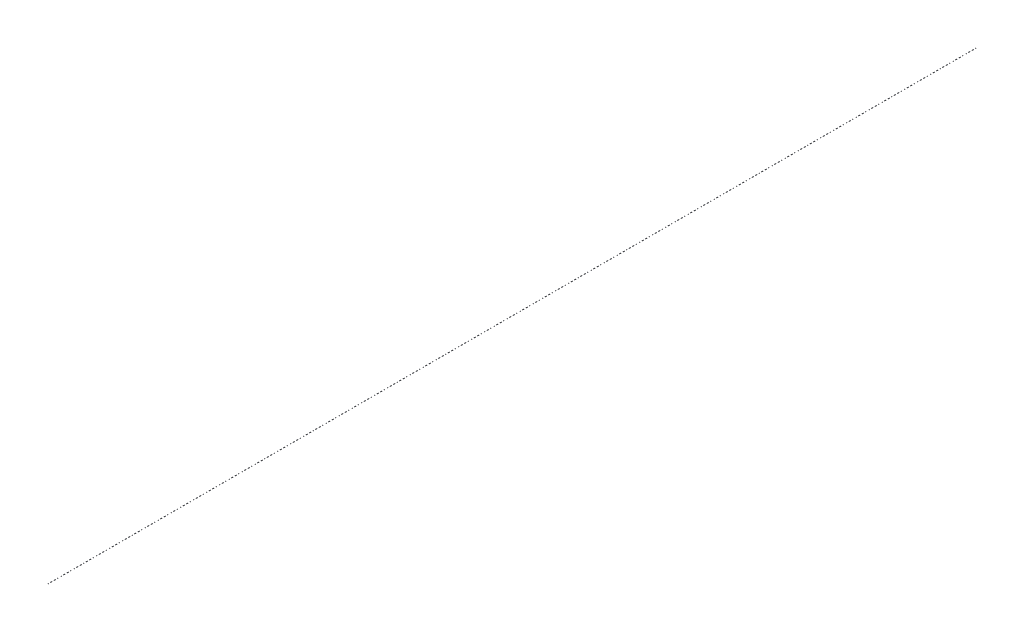
SolidWorks part; units mm, degrees
ref_plane "Front Plane" through (0, 0, 0) normal (0, 0, 1) x (1, 0, 0)
ref_plane "Top Plane" through (0, 0, 0) normal (0, 1, 0) x (1, 0, 0)
ref_plane "Right Plane" through (0, 0, 0) normal (1, 0, 0) x (0, 0, -1)
sketch "Sketch1" plane through (0, 0, 0) normal (0, 0, 1) x (1, 0, 0)
  circle A0 centre (0, 0) radius 0.075
  circle A1 centre (0, 0) radius 0.0625
  dimension "D1" = 0.125
  dimension "D2" = 0.15
extrude "Boss-Extrude1" add sketch "Sketch1" along normal blind 1900
